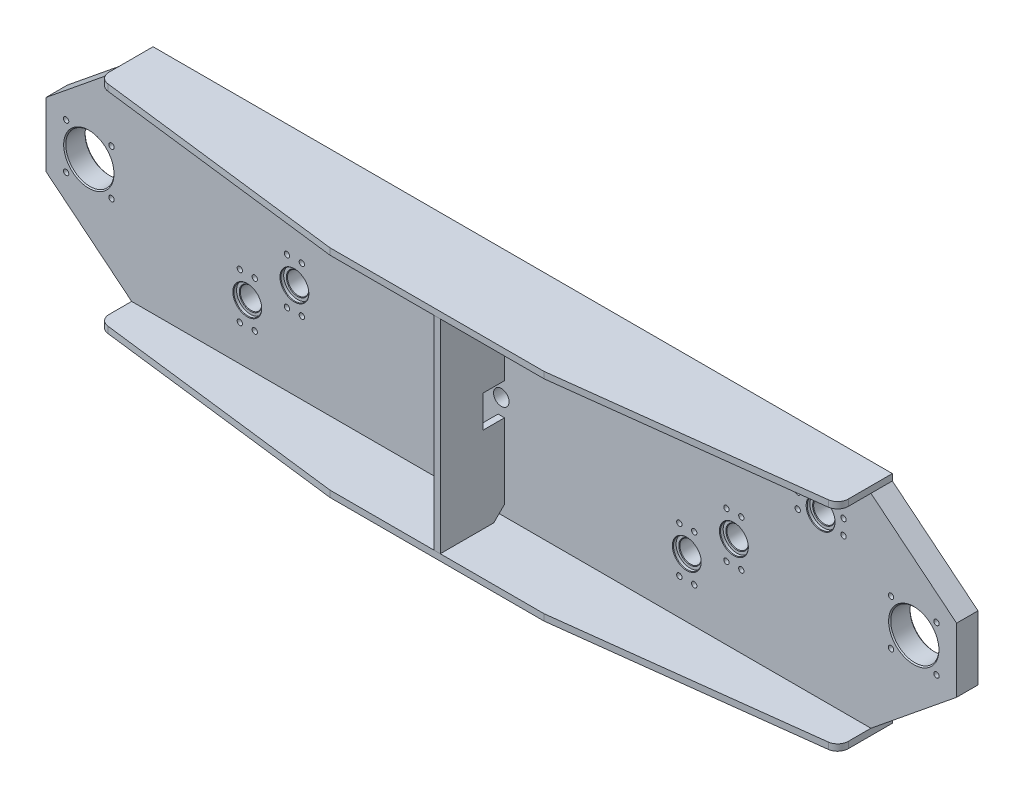
from build123d import *

# Parameters (mm, degrees)
SKETCH1_W                  = 280
SKETCH1_H                  = 350
BOSS_EXTRUDE1_DEPTH        = 20
CUT_EXTRUDE4_REACH         = 227
SKETCH8_R                  = 10
SKETCH9_R                  = 13
CUT_EXTRUDE5_DEPTH         = 3
CHAMFER3_SIZE              = 0.5
CUT_EXTRUDE6_REACH         = 227
SKETCH10_R                 = 10
SKETCH11_R                 = 13
CUT_EXTRUDE7_DEPTH         = 3
CHAMFER4_SIZE              = 0.5
SKETCH13_OUTSIDE_W         = 371.732
SKETCH13_OUTSIDE_H         = 441.732
SKETCH13_OUTSIDE_W_2       = 451.333436131
SKETCH13_OUTSIDE_H_2       = 190
CUT_EXTRUDE8_DEPTH         = 226
LPATTERN1_COUNT            = 2
LPATTERN1_PITCH            = 410.5
SKETCH14_W                 = 20
SKETCH14_H                 = 190
BOSS_EXTRUDE2_DEPTH        = 130.5
BOSS_EXTRUDE3_DEPTH        = 20
CUT_EXTRUDE9_REACH         = 579.992
SKETCH16_R                 = 22.5
CHAMFER5_SIZE              = 1
CHAMFER5_OF_MIRROR1_SIZE   = 1
M16X1_5_TAPPED_HOLE1_D     = 14.5
BOSS_EXTRUDE4_DEPTH        = 6
FILLET1_R                  = 10
BOSS_EXTRUDE5_DEPTH        = 3
BOSS_EXTRUDE5_DEPTH_BACK   = 3
SKETCH20_W                 = 20
SKETCH20_H                 = 30
CUT_EXTRUDE10_DEPTH        = 6
CIRPATTERN2_COUNT          = 10
LPATTERN6_COUNT            = 2
LPATTERN6_PITCH            = 410.5
LPATTERN7_COUNT            = 2
LPATTERN7_PITCH            = 44
LPATTERN7_COUNT_DIR2       = 2
LPATTERN7_PITCH_DIR2       = 34
CIRPATTERN3_COUNT          = 10
LPATTERN8_COUNT            = 2
LPATTERN8_PITCH            = 101
LPATTERN8_COUNT_DIR2       = 2
LPATTERN8_PITCH_DIR2       = 20
LPATTERN12_COUNT           = 2
LPATTERN12_PITCH           = 410.5
SKETCH24_W                 = 2.5
SKETCH24_H                 = 20
CIRPATTERN4_COUNT          = 4
LPATTERN13_COUNT           = 2
LPATTERN13_PITCH           = 770.5
LPATTERN13_COPY_1_SKETCH_W = 2.5
LPATTERN13_COPY_1_SKETCH_H = 20
LPATTERN13_COPY_2_SKETCH_W = 2.5
LPATTERN13_COPY_2_SKETCH_H = 20
LPATTERN13_COPY_3_SKETCH_W = 2.5
LPATTERN13_COPY_3_SKETCH_H = 20


with BuildPart() as part:
    # Sketch1 → Boss-Extrude1 (new body)
    with BuildSketch(Plane.XY):
        Rectangle(SKETCH1_W, SKETCH1_H)
    extrude(amount=BOSS_EXTRUDE1_DEPTH)

    # Sketch8 → Cut-Extrude4 (cut, up to next)
    with BuildSketch(Plane.XY.offset(20), mode=Mode.PRIVATE) as cut_extrude4_sk1:
        with Locations((-32, -120)):
            Circle(SKETCH8_R)
    cut_extrude4_tool1 = extrude(cut_extrude4_sk1.sketch, amount=-CUT_EXTRUDE4_REACH, mode=Mode.PRIVATE) & part.part
    # Sketch8 → Cut-Extrude4 (cut, up to next)
    with BuildSketch(Plane.XY.offset(20), mode=Mode.PRIVATE) as cut_extrude4_sk2:
        with Locations((12, -86)):
            Circle(SKETCH8_R)
    cut_extrude4_tool2 = extrude(cut_extrude4_sk2.sketch, amount=-CUT_EXTRUDE4_REACH, mode=Mode.PRIVATE) & part.part
    # Sketch8 → Cut-Extrude4 (cut, up to next)
    with BuildSketch(Plane.XY.offset(20), mode=Mode.PRIVATE) as cut_extrude4_sk3:
        with Locations((-8, -5)):
            Circle(SKETCH8_R)
    cut_extrude4_tool3 = extrude(cut_extrude4_sk3.sketch, amount=-CUT_EXTRUDE4_REACH, mode=Mode.PRIVATE) & part.part
    # Sketch8 → Cut-Extrude4 (cut, up to next)
    with BuildSketch(Plane.XY.offset(20), mode=Mode.PRIVATE) as cut_extrude4_sk4:
        with Locations((93, -25)):
            Circle(SKETCH8_R)
    cut_extrude4_tool4 = extrude(cut_extrude4_sk4.sketch, amount=-CUT_EXTRUDE4_REACH, mode=Mode.PRIVATE) & part.part
    add(cut_extrude4_tool1.solids().sort_by_distance((-32, -120, 20))[0], mode=Mode.SUBTRACT)
    add(cut_extrude4_tool2.solids().sort_by_distance((12, -86, 20))[0], mode=Mode.SUBTRACT)
    add(cut_extrude4_tool3.solids().sort_by_distance((-8, -5, 20))[0], mode=Mode.SUBTRACT)
    add(cut_extrude4_tool4.solids().sort_by_distance((93, -25, 20))[0], mode=Mode.SUBTRACT)

    # Sketch9 → Cut-Extrude5 (cut)
    with BuildSketch(Plane.XY.offset(20)):
        with Locations((-32, -120)):
            Circle(SKETCH9_R)
        with Locations((12, -86)):
            Circle(SKETCH9_R)
        with Locations((93, -25)):
            Circle(SKETCH9_R)
        with Locations((-8, -5)):
            Circle(SKETCH9_R)
    extrude(amount=-CUT_EXTRUDE5_DEPTH, mode=Mode.SUBTRACT)

    # Chamfer3
    chamfer3_edges = [part.edges().sort_by_distance(p)[0] for p in [
        (-42, -120, 0),
        (2, -86, 0),
        (-18, -5, 0),
        (83, -25, 0),
        (-42, -120, 17),
        (2, -86, 17),
        (83, -25, 17),
        (-18, -5, 17),
    ]]
    chamfer(chamfer3_edges, length=CHAMFER3_SIZE)

    # Sketch10 → Cut-Extrude6 (cut, up to next)
    with BuildSketch(Plane.XY.offset(20), mode=Mode.PRIVATE) as cut_extrude6_sk1:
        with Locations((-66, 92)):
            Circle(SKETCH10_R)
    cut_extrude6_tool1 = extrude(cut_extrude6_sk1.sketch, amount=-CUT_EXTRUDE6_REACH, mode=Mode.PRIVATE) & part.part
    # Sketch10 → Cut-Extrude6 (cut, up to next)
    with BuildSketch(Plane.XY.offset(20), mode=Mode.PRIVATE) as cut_extrude6_sk2:
        with Locations((-102, 104)):
            Circle(SKETCH10_R)
    cut_extrude6_tool2 = extrude(cut_extrude6_sk2.sketch, amount=-CUT_EXTRUDE6_REACH, mode=Mode.PRIVATE) & part.part
    # Sketch10 → Cut-Extrude6 (cut, up to next)
    with BuildSketch(Plane.XY.offset(20), mode=Mode.PRIVATE) as cut_extrude6_sk3:
        with Locations((-2, 58)):
            Circle(SKETCH10_R)
    cut_extrude6_tool3 = extrude(cut_extrude6_sk3.sketch, amount=-CUT_EXTRUDE6_REACH, mode=Mode.PRIVATE) & part.part
    # Sketch10 → Cut-Extrude6 (cut, up to next)
    with BuildSketch(Plane.XY.offset(20), mode=Mode.PRIVATE) as cut_extrude6_sk4:
        with Locations((57, 34)):
            Circle(SKETCH10_R)
    cut_extrude6_tool4 = extrude(cut_extrude6_sk4.sketch, amount=-CUT_EXTRUDE6_REACH, mode=Mode.PRIVATE) & part.part
    add(cut_extrude6_tool1.solids().sort_by_distance((-66, 92, 20))[0], mode=Mode.SUBTRACT)
    add(cut_extrude6_tool2.solids().sort_by_distance((-102, 104, 20))[0], mode=Mode.SUBTRACT)
    add(cut_extrude6_tool3.solids().sort_by_distance((-2, 58, 20))[0], mode=Mode.SUBTRACT)
    add(cut_extrude6_tool4.solids().sort_by_distance((57, 34, 20))[0], mode=Mode.SUBTRACT)

    # Sketch11 → Cut-Extrude7 (cut)
    with BuildSketch(Plane.XY.offset(20)):
        with Locations((-102, 104)):
            Circle(SKETCH11_R)
        with Locations((-66, 92)):
            Circle(SKETCH11_R)
        with Locations((-2, 58)):
            Circle(SKETCH11_R)
        with Locations((57, 34)):
            Circle(SKETCH11_R)
    extrude(amount=-CUT_EXTRUDE7_DEPTH, mode=Mode.SUBTRACT)

    # Chamfer4
    chamfer4_edges = [part.edges().sort_by_distance(p)[0] for p in [
        (-79, 92, 20),
        (-76, 92, 17),
        (-15, 58, 20),
        (-12, 58, 17),
        (44, 34, 20),
        (47, 34, 17),
        (-45, -120, 20),
        (-1, -86, 20),
        (80, -25, 20),
        (-21, -5, 20),
        (-76, 92, 0),
        (-112, 104, 0),
        (-12, 58, 0),
        (47, 34, 0),
        (-115, 104, 20),
        (-112, 104, 17),
    ]]
    chamfer(chamfer4_edges, length=CHAMFER4_SIZE)

    # Sketch13 outside → Cut-Extrude8 (cut, through all)
    with BuildSketch(Plane.XY.offset(20)):
        Rectangle(SKETCH13_OUTSIDE_W, SKETCH13_OUTSIDE_H)
        with Locations((13.549536937, -80)):
            Rectangle(SKETCH13_OUTSIDE_W_2, SKETCH13_OUTSIDE_H_2, mode=Mode.SUBTRACT)
    extrude(amount=-CUT_EXTRUDE8_DEPTH, mode=Mode.SUBTRACT)


with BuildPart() as lpattern1_1:
    # LPattern1: pattern copy
    add(part.part.moved(Location(Vector(1, 0, 0) * (1 * LPATTERN1_PITCH))))


with BuildPart() as part_1:
    add(part.part)

    add(lpattern1_1.part)  # Boss-Extrude2 merges LPattern1_1
    # Sketch14 → Boss-Extrude2 (add)
    with BuildSketch(Plane(origin=(140, 0, 0), x_dir=(0, 0, -1), z_dir=(1, 0, 0))):
        with Locations((-10, -80)):
            Rectangle(SKETCH14_W, SKETCH14_H)
    extrude(amount=BOSS_EXTRUDE2_DEPTH)

    # Sketch15 → Boss-Extrude3 (add)
    with BuildSketch(Plane.XY.offset(20)):
        Polygon((-140, 15), (-220, -50), (-220, -110), (-140, -175), align=None)
    boss_extrude3 = extrude(amount=-BOSS_EXTRUDE3_DEPTH)

    # Sketch16 → Cut-Extrude9 (cut, up to next)
    with BuildSketch(Plane.XY.offset(20), mode=Mode.PRIVATE) as cut_extrude9_sk1:
        with Locations((-180, -80)):
            Circle(SKETCH16_R)
    cut_extrude9_tool1 = extrude(cut_extrude9_sk1.sketch, amount=-CUT_EXTRUDE9_REACH, mode=Mode.PRIVATE) & part_1.part
    cut_extrude9 = cut_extrude9_tool1.solids().sort_by_distance((-180, -80, 20))[0]
    add(cut_extrude9, mode=Mode.SUBTRACT)

    # Chamfer5
    chamfer5_edges = [part_1.edges().sort_by_distance(p)[0] for p in [
        (-202.5, -80, 20),
        (-202.5, -80, 0),
    ]]
    chamfer(chamfer5_edges, length=CHAMFER5_SIZE)

    # Mirror1: Boss-Extrude3, Cut-Extrude9 across plane
    add(boss_extrude3.mirror(Plane.ZY.offset(-205.25)))
    add(cut_extrude9.mirror(Plane.ZY.offset(-205.25)), mode=Mode.SUBTRACT)

    # Chamfer5 of Mirror1
    chamfer5_of_mirror1_edges = [part_1.edges().sort_by_distance(p)[0] for p in [
        (613, -80, 20),
        (613, -80, 0),
    ]]
    chamfer(chamfer5_of_mirror1_edges, length=CHAMFER5_OF_MIRROR1_SIZE)

    # M16x1.5 Tapped Hole1 (through all)
    with Locations(Plane(origin=(205.25, -80, 20), x_dir=(1, 0, 0), z_dir=(0, 0, 1))):
        with Locations((0, 0)):
            Hole(M16X1_5_TAPPED_HOLE1_D / 2)

    # Sketch22 → M6 Tapped Hole1 (revolve, cut)
    with BuildSketch(Plane(origin=(-38.952882373, -98.601228383, 20), x_dir=(0, -1, 0), z_dir=(1, 0, 0))):
        Polygon((0, 0), (0, 18.502151548), (2.5, 17), (2.5, 0), align=None)
    m6_tapped_hole1 = revolve(axis=Axis((-38.952882373, -98.601228383, 26.35), (0, 0, -1)), mode=Mode.SUBTRACT)

    # CirPattern2: M6 Tapped Hole1 ×10 about axis, 6 skipped
    cirpattern2_axis = Axis((-32, -120, 0), (0, 0, -1))
    add([m6_tapped_hole1.rotate(cirpattern2_axis, i * 360 / CIRPATTERN2_COUNT) for i in range(1, CIRPATTERN2_COUNT) if i not in (2, 3, 4, 7, 8, 9)], mode=Mode.SUBTRACT)

    # LPattern6: M6 Tapped Hole1 ×2
    with Locations(*[(i * LPATTERN6_PITCH, 0, 0) for i in range(1, LPATTERN6_COUNT)]):
        add(m6_tapped_hole1, mode=Mode.SUBTRACT)

    # LPattern6 copy 1 sketch → LPattern6 copy 1 (revolve, cut)
    with BuildSketch(Plane(origin=(385.452882373, -98.601228383, 20), x_dir=(-0.5877852522924731, -0.8090169943749475, 0), z_dir=(0.8090169943749475, -0.5877852522924731, 0))):
        Polygon((0, 0), (0, 18.502151548), (2.5, 17), (2.5, 0), align=None)
    revolve(axis=Axis((385.452882373, -98.601228383, 26.35), (0, 0, -1)), mode=Mode.SUBTRACT)

    # LPattern6 copy 2 sketch → LPattern6 copy 2 (revolve, cut)
    with BuildSketch(Plane(origin=(385.452882373, -141.398771617, 20), x_dir=(0, 1, 0), z_dir=(-1, 0, 0))):
        Polygon((0, 0), (0, 18.502151548), (2.5, 17), (2.5, 0), align=None)
    revolve(axis=Axis((385.452882373, -141.398771617, 26.35), (0, 0, -1)), mode=Mode.SUBTRACT)

    # LPattern6 copy 3 sketch → LPattern6 copy 3 (revolve, cut)
    with BuildSketch(Plane(origin=(371.547117627, -141.398771617, 20), x_dir=(0.587785252292473, 0.8090169943749476, 0), z_dir=(-0.8090169943749476, 0.587785252292473, 0))):
        Polygon((0, 0), (0, 18.502151548), (2.5, 17), (2.5, 0), align=None)
    revolve(axis=Axis((371.547117627, -141.398771617, 26.35), (0, 0, -1)), mode=Mode.SUBTRACT)

    # LPattern7: M6 Tapped Hole1 2 × 2, 2 skipped
    with Locations(*[(i * LPATTERN7_PITCH, j * LPATTERN7_PITCH_DIR2, 0) for i in range(LPATTERN7_COUNT) for j in range(LPATTERN7_COUNT_DIR2) if (i, j) not in ((0, 0), (0, 1), (1, 0))]):
        add(m6_tapped_hole1, mode=Mode.SUBTRACT)

    # LPattern7 copy 1 sketch → LPattern7 copy 1 (revolve, cut)
    with BuildSketch(Plane(origin=(18.952882373, -64.601228383, 20), x_dir=(-0.5877852522924731, -0.8090169943749475, 0), z_dir=(0.8090169943749475, -0.5877852522924731, 0))):
        Polygon((0, 0), (0, 18.502151548), (2.5, 17), (2.5, 0), align=None)
    revolve(axis=Axis((18.952882373, -64.601228383, 26.35), (0, 0, -1)), mode=Mode.SUBTRACT)

    # LPattern7 copy 2 sketch → LPattern7 copy 2 (revolve, cut)
    with BuildSketch(Plane(origin=(18.952882373, -107.398771617, 20), x_dir=(0, 1, 0), z_dir=(-1, 0, 0))):
        Polygon((0, 0), (0, 18.502151548), (2.5, 17), (2.5, 0), align=None)
    revolve(axis=Axis((18.952882373, -107.398771617, 26.35), (0, 0, -1)), mode=Mode.SUBTRACT)

    # LPattern7 copy 3 sketch → LPattern7 copy 3 (revolve, cut)
    with BuildSketch(Plane(origin=(5.047117627, -107.398771617, 20), x_dir=(0.587785252292473, 0.8090169943749476, 0), z_dir=(-0.8090169943749476, 0.587785252292473, 0))):
        Polygon((0, 0), (0, 18.502151548), (2.5, 17), (2.5, 0), align=None)
    revolve(axis=Axis((5.047117627, -107.398771617, 26.35), (0, 0, -1)), mode=Mode.SUBTRACT)

    # Sketch23 → M6 Tapped Hole2 (revolve, cut)
    with BuildSketch(Plane(origin=(-29.398771617, -11.952882373, 20), x_dir=(0, -1, 0), z_dir=(1, 0, 0))):
        Polygon((0, 0), (0, 18.502151548), (2.5, 17), (2.5, 0), align=None)
    m6_tapped_hole2 = revolve(axis=Axis((-29.398771617, -11.952882373, 26.35), (0, 0, -1)), mode=Mode.SUBTRACT)

    # CirPattern3: M6 Tapped Hole2 ×10 about axis, 6 skipped
    cirpattern3_axis = Axis((-8, -5, 0), (0, 0, -1))
    add([m6_tapped_hole2.rotate(cirpattern3_axis, i * 360 / CIRPATTERN3_COUNT) for i in range(1, CIRPATTERN3_COUNT) if i not in (2, 3, 4, 7, 8, 9)], mode=Mode.SUBTRACT)

    # LPattern8: M6 Tapped Hole2 2 × 2, 2 skipped
    with Locations(*[(i * LPATTERN8_PITCH, -j * LPATTERN8_PITCH_DIR2, 0) for i in range(LPATTERN8_COUNT) for j in range(LPATTERN8_COUNT_DIR2) if (i, j) not in ((0, 0), (0, 1), (1, 0))]):
        add(m6_tapped_hole2, mode=Mode.SUBTRACT)

    # LPattern8 copy 1 sketch → LPattern8 copy 1 (revolve, cut)
    with BuildSketch(Plane(origin=(71.601228383, -18.047117627, 20), x_dir=(-0.5877852522924731, -0.8090169943749475, 0), z_dir=(0.8090169943749475, -0.5877852522924731, 0))):
        Polygon((0, 0), (0, 18.502151548), (2.5, 17), (2.5, 0), align=None)
    revolve(axis=Axis((71.601228383, -18.047117627, 26.35), (0, 0, -1)), mode=Mode.SUBTRACT)

    # LPattern8 copy 2 sketch → LPattern8 copy 2 (revolve, cut)
    with BuildSketch(Plane(origin=(114.398771617, -18.047117627, 20), x_dir=(0, 1, 0), z_dir=(-1, 0, 0))):
        Polygon((0, 0), (0, 18.502151548), (2.5, 17), (2.5, 0), align=None)
    revolve(axis=Axis((114.398771617, -18.047117627, 26.35), (0, 0, -1)), mode=Mode.SUBTRACT)

    # LPattern8 copy 3 sketch → LPattern8 copy 3 (revolve, cut)
    with BuildSketch(Plane(origin=(114.398771617, -31.952882373, 20), x_dir=(0.587785252292473, 0.8090169943749476, 0), z_dir=(-0.8090169943749476, 0.587785252292473, 0))):
        Polygon((0, 0), (0, 18.502151548), (2.5, 17), (2.5, 0), align=None)
    revolve(axis=Axis((114.398771617, -31.952882373, 26.35), (0, 0, -1)), mode=Mode.SUBTRACT)

    # LPattern12: M6 Tapped Hole2 ×2
    with Locations(*[(i * LPATTERN12_PITCH, 0, 0) for i in range(1, LPATTERN12_COUNT)]):
        add(m6_tapped_hole2, mode=Mode.SUBTRACT)

    # LPattern12 copy 1 sketch → LPattern12 copy 1 (revolve, cut)
    with BuildSketch(Plane(origin=(415.547117627, -64.601228383, 20), x_dir=(0, -1, 0), z_dir=(1, 0, 0))):
        Polygon((0, 0), (0, 18.502151548), (2.5, 17), (2.5, 0), align=None)
    revolve(axis=Axis((415.547117627, -64.601228383, 26.35), (0, 0, -1)), mode=Mode.SUBTRACT)

    # LPattern12 copy 2 sketch → LPattern12 copy 2 (revolve, cut)
    with BuildSketch(Plane(origin=(429.452882373, -64.601228383, 20), x_dir=(-0.5877852522924731, -0.8090169943749475, 0), z_dir=(0.8090169943749475, -0.5877852522924731, 0))):
        Polygon((0, 0), (0, 18.502151548), (2.5, 17), (2.5, 0), align=None)
    revolve(axis=Axis((429.452882373, -64.601228383, 26.35), (0, 0, -1)), mode=Mode.SUBTRACT)

    # LPattern12 copy 3 sketch → LPattern12 copy 3 (revolve, cut)
    with BuildSketch(Plane(origin=(429.452882373, -107.398771617, 20), x_dir=(0, 1, 0), z_dir=(-1, 0, 0))):
        Polygon((0, 0), (0, 18.502151548), (2.5, 17), (2.5, 0), align=None)
    revolve(axis=Axis((429.452882373, -107.398771617, 26.35), (0, 0, -1)), mode=Mode.SUBTRACT)

    # LPattern12 copy 4 sketch → LPattern12 copy 4 (revolve, cut)
    with BuildSketch(Plane(origin=(415.547117627, -107.398771617, 20), x_dir=(0.587785252292473, 0.8090169943749476, 0), z_dir=(-0.8090169943749476, 0.587785252292473, 0))):
        Polygon((0, 0), (0, 18.502151548), (2.5, 17), (2.5, 0), align=None)
    revolve(axis=Axis((415.547117627, -107.398771617, 26.35), (0, 0, -1)), mode=Mode.SUBTRACT)

    # LPattern12 copy 5 sketch → LPattern12 copy 5 (revolve, cut)
    with BuildSketch(Plane(origin=(381.101228383, 1.952882373, 20), x_dir=(-0.5877852522924731, -0.8090169943749475, 0), z_dir=(0.8090169943749475, -0.5877852522924731, 0))):
        Polygon((0, 0), (0, 18.502151548), (2.5, 17), (2.5, 0), align=None)
    revolve(axis=Axis((381.101228383, 1.952882373, 26.35), (0, 0, -1)), mode=Mode.SUBTRACT)

    # LPattern12 copy 6 sketch → LPattern12 copy 6 (revolve, cut)
    with BuildSketch(Plane(origin=(423.898771617, 1.952882373, 20), x_dir=(0, 1, 0), z_dir=(-1, 0, 0))):
        Polygon((0, 0), (0, 18.502151548), (2.5, 17), (2.5, 0), align=None)
    revolve(axis=Axis((423.898771617, 1.952882373, 26.35), (0, 0, -1)), mode=Mode.SUBTRACT)

    # LPattern12 copy 7 sketch → LPattern12 copy 7 (revolve, cut)
    with BuildSketch(Plane(origin=(423.898771617, -11.952882373, 20), x_dir=(0.587785252292473, 0.8090169943749476, 0), z_dir=(-0.8090169943749476, 0.587785252292473, 0))):
        Polygon((0, 0), (0, 18.502151548), (2.5, 17), (2.5, 0), align=None)
    revolve(axis=Axis((423.898771617, -11.952882373, 26.35), (0, 0, -1)), mode=Mode.SUBTRACT)

    # LPattern12 copy 8 sketch → LPattern12 copy 8 (revolve, cut)
    with BuildSketch(Plane(origin=(482.101228383, -31.952882373, 20), x_dir=(0, -1, 0), z_dir=(1, 0, 0))):
        Polygon((0, 0), (0, 18.502151548), (2.5, 17), (2.5, 0), align=None)
    revolve(axis=Axis((482.101228383, -31.952882373, 26.35), (0, 0, -1)), mode=Mode.SUBTRACT)

    # LPattern12 copy 9 sketch → LPattern12 copy 9 (revolve, cut)
    with BuildSketch(Plane(origin=(482.101228383, -18.047117627, 20), x_dir=(-0.5877852522924731, -0.8090169943749475, 0), z_dir=(0.8090169943749475, -0.5877852522924731, 0))):
        Polygon((0, 0), (0, 18.502151548), (2.5, 17), (2.5, 0), align=None)
    revolve(axis=Axis((482.101228383, -18.047117627, 26.35), (0, 0, -1)), mode=Mode.SUBTRACT)

    # LPattern12 copy 10 sketch → LPattern12 copy 10 (revolve, cut)
    with BuildSketch(Plane(origin=(524.898771617, -18.047117627, 20), x_dir=(0, 1, 0), z_dir=(-1, 0, 0))):
        Polygon((0, 0), (0, 18.502151548), (2.5, 17), (2.5, 0), align=None)
    revolve(axis=Axis((524.898771617, -18.047117627, 26.35), (0, 0, -1)), mode=Mode.SUBTRACT)

    # LPattern12 copy 11 sketch → LPattern12 copy 11 (revolve, cut)
    with BuildSketch(Plane(origin=(524.898771617, -31.952882373, 20), x_dir=(0.587785252292473, 0.8090169943749476, 0), z_dir=(-0.8090169943749476, 0.587785252292473, 0))):
        Polygon((0, 0), (0, 18.502151548), (2.5, 17), (2.5, 0), align=None)
    revolve(axis=Axis((524.898771617, -31.952882373, 26.35), (0, 0, -1)), mode=Mode.SUBTRACT)

    # Sketch24 → M6 Tapped Hole3 (revolve, cut)
    with BuildSketch(Plane(origin=(-158.786796564, -58.786796564, 20), x_dir=(0, -1, 0), z_dir=(1, 0, 0))):
        with Locations((1.25, 10)):
            Rectangle(SKETCH24_W, SKETCH24_H)
    m6_tapped_hole3 = revolve(axis=Axis((-158.786796564, -58.786796564, 26.35), (0, 0, -1)), mode=Mode.SUBTRACT)

    # CirPattern4: M6 Tapped Hole3 ×4 about axis
    cirpattern4_axis = Axis((-180, -80, 0), (0, 0, 1))
    for i in range(1, CIRPATTERN4_COUNT):
        add(m6_tapped_hole3.rotate(cirpattern4_axis, i * 360 / CIRPATTERN4_COUNT), mode=Mode.SUBTRACT)

    # LPattern13: M6 Tapped Hole3 ×2
    with Locations(*[(i * LPATTERN13_PITCH, 0, 0) for i in range(1, LPATTERN13_COUNT)]):
        add(m6_tapped_hole3, mode=Mode.SUBTRACT)

    # LPattern13 copy 1 sketch → LPattern13 copy 1 (revolve, cut)
    with BuildSketch(Plane(origin=(569.286796564, -58.786796564, 20), x_dir=(1, 0, 0), z_dir=(0, 1, 0))):
        with Locations((1.25, 10)):
            Rectangle(LPATTERN13_COPY_1_SKETCH_W, LPATTERN13_COPY_1_SKETCH_H)
    revolve(axis=Axis((569.286796564, -58.786796564, 26.35), (0, 0, -1)), mode=Mode.SUBTRACT)

    # LPattern13 copy 2 sketch → LPattern13 copy 2 (revolve, cut)
    with BuildSketch(Plane(origin=(569.286796564, -101.213203436, 20), x_dir=(0, 1, 0), z_dir=(-1, 0, 0))):
        with Locations((1.25, 10)):
            Rectangle(LPATTERN13_COPY_2_SKETCH_W, LPATTERN13_COPY_2_SKETCH_H)
    revolve(axis=Axis((569.286796564, -101.213203436, 26.35), (0, 0, -1)), mode=Mode.SUBTRACT)

    # LPattern13 copy 3 sketch → LPattern13 copy 3 (revolve, cut)
    with BuildSketch(Plane(origin=(611.713203436, -101.213203436, 20), x_dir=(-1, 0, 0), z_dir=(0, -1, 0))):
        with Locations((1.25, 10)):
            Rectangle(LPATTERN13_COPY_3_SKETCH_W, LPATTERN13_COPY_3_SKETCH_H)
    revolve(axis=Axis((611.713203436, -101.213203436, 26.35), (0, 0, -1)), mode=Mode.SUBTRACT)


with BuildPart() as body_2:
    # Sketch18 → Boss-Extrude4 (new body)
    with BuildSketch(Plane.XZ.offset(175)):
        Polygon((-140, 0), (-140, 50), (105.25, 80), (305.25, 80), (550.5, 50), (550.5, 0), align=None)
    extrude(amount=BOSS_EXTRUDE4_DEPTH)

    # Fillet1
    fillet1_edges = [body_2.edges().sort_by_distance(p)[0] for p in [
        (-140, -178, 50),
        (550.5, -178, 50),
    ]]
    fillet(fillet1_edges, radius=FILLET1_R)


with BuildPart() as body_3:
    # Mirror2: mirrored copy
    add(body_2.part.mirror(Plane(origin=(0, -80, 0), x_dir=(0, 0, 1), z_dir=(0, -1, 0))))


with BuildPart() as body_4:
    # Sketch19 → Boss-Extrude5 (new, two sides: drawn at the far end of the back side and taken through both)
    with BuildSketch(Plane.ZY.offset(-205.25).offset(-BOSS_EXTRUDE5_DEPTH_BACK)):
        Polygon((80, 15), (30, 15), (20, 5), (20, -165), (30, -175), (80, -175), align=None)
    extrude(amount=BOSS_EXTRUDE5_DEPTH + BOSS_EXTRUDE5_DEPTH_BACK)

    # Sketch20 → Cut-Extrude10 (cut)
    with BuildSketch(Plane.ZY.offset(-202.25)):
        with Locations((30, -80)):
            Rectangle(SKETCH20_W, SKETCH20_H)
    extrude(amount=-CUT_EXTRUDE10_DEPTH, mode=Mode.SUBTRACT)


solid = Compound([part_1.part, body_2.part, body_3.part, body_4.part])
